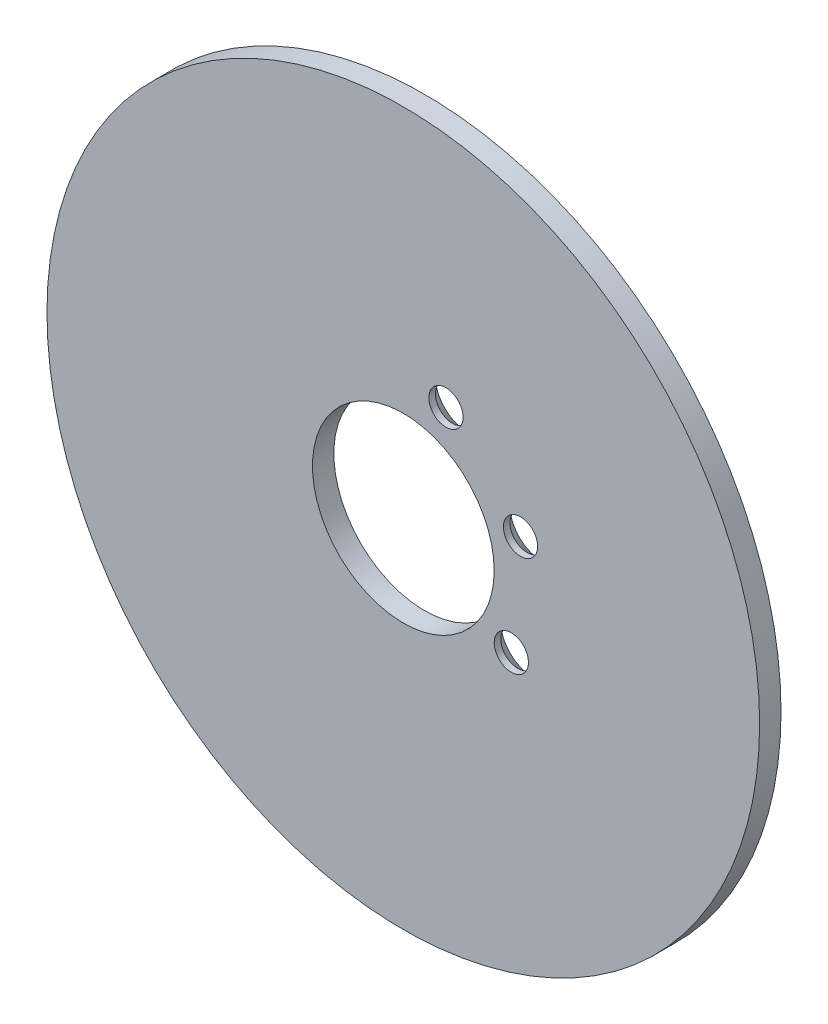
from build123d import *

# Parameters (mm, degrees)
SKETCH1_R                                    = 50
SKETCH1_R_2                                  = 12.75
BOSS_EXTRUDE1_DEPTH                          = 3
CSK_FOR_M4_HEX_SOCKET_COUNTERSUNK_CA_2_COUNT = 2
CSK_FOR_M4_HEX_SOCKET_COUNTERSUNK_CA_2_PITCH = 26.811555509
CSK_FOR_M4_HEX_SOCKET_COUNTERSUNK_CA_3_COUNT = 2
CSK_FOR_M4_HEX_SOCKET_COUNTERSUNK_CA_3_PITCH = 14.791639161


with BuildPart() as part:
    # Sketch1 → Boss-Extrude1 (new body)
    with BuildSketch(Plane.XY):
        Circle(SKETCH1_R)
        Circle(SKETCH1_R_2, mode=Mode.SUBTRACT)
    extrude(amount=BOSS_EXTRUDE1_DEPTH)

    # Sketch2 → CSK for M4 Hex Socket Countersunk Cap Screw1 (revolve, cut)
    with BuildSketch(Plane(origin=(5.985352508, 16.444620864, 0), x_dir=(0, 1, 0), z_dir=(1, 0, 0))):
        Polygon((0, 0), (0, 3), (2.4, 3), (2.4, 2.08), (4.48, 0), align=None)
    csk_for_m4_hex_socket_countersunk_cap_sc = revolve(axis=Axis((5.985352508, 16.444620864, -6.35), (0, 0, 1)), mode=Mode.SUBTRACT)

    # CSK for M4 Hex Socket Countersunk Ca 2: CSK for M4 Hex Socket Countersunk Cap Screw1 ×2
    with Locations(*[Vector(0.3420201433256698, -0.9396926207859081, 0) * (i * CSK_FOR_M4_HEX_SOCKET_COUNTERSUNK_CA_2_PITCH) for i in range(1, CSK_FOR_M4_HEX_SOCKET_COUNTERSUNK_CA_2_COUNT)]):
        add(csk_for_m4_hex_socket_countersunk_cap_sc, mode=Mode.SUBTRACT)

    # CSK for M4 Hex Socket Countersunk Ca 3: CSK for M4 Hex Socket Countersunk Cap Screw1 ×2
    with Locations(*[Vector(0.7071067811865491, -0.707106781186546, 0) * (i * CSK_FOR_M4_HEX_SOCKET_COUNTERSUNK_CA_3_PITCH) for i in range(1, CSK_FOR_M4_HEX_SOCKET_COUNTERSUNK_CA_3_COUNT)]):
        add(csk_for_m4_hex_socket_countersunk_cap_sc, mode=Mode.SUBTRACT)


solid = part.part
